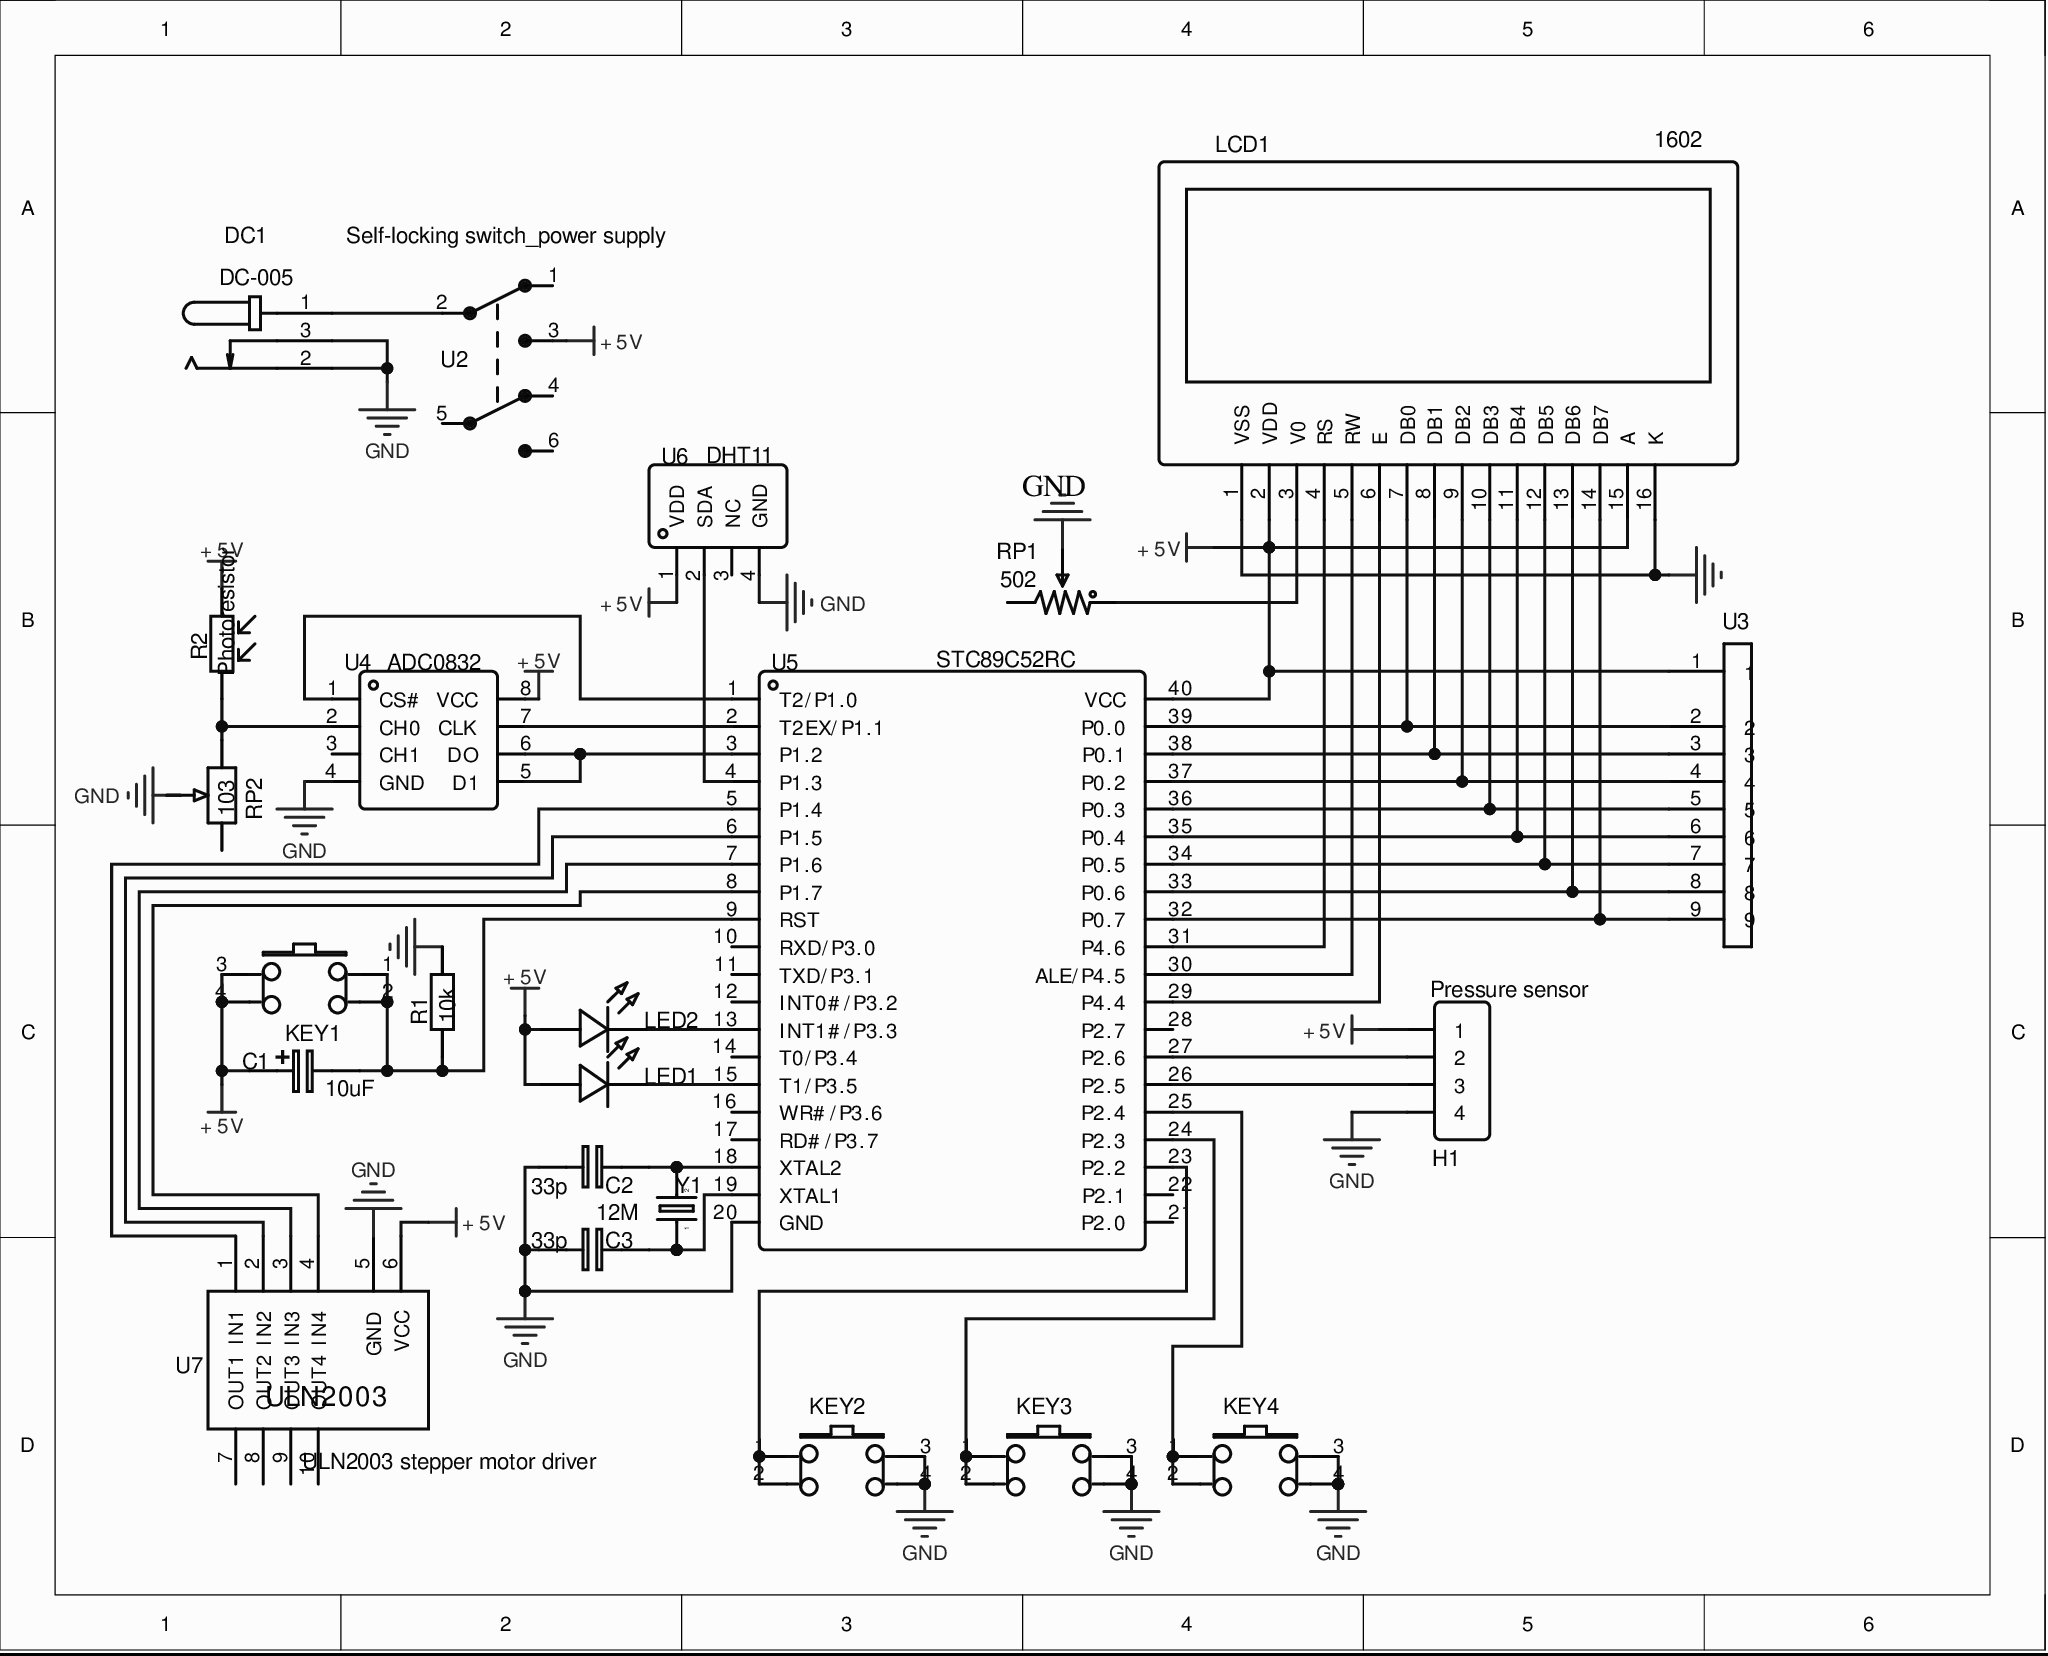
[diagram p0: MISC80828-9.schdoc]
# Altium project MISC80828-7.PrjPcb
1 sheet, 23 parts. Net scope: global (net labels, ports and power ports of the same name join across sheets).
Board file: MISC80828.PcbDoc

## Sheet MISC80828-9.schdoc
size 188 x 152 mm

### Parts
C1  10uF  [RB7.6-15]
C2  33p  [RAD-0.1]
C3  33p  [RAD-0.1]
DC1  DC-005  [DC-005]
H1  Pressure sensor  [HDR1X4]
KEY1  button6*6*8.5  [四脚轻触开关]  (value not drawn)
KEY2  button6*6*8.5  [四脚轻触开关]  (value not drawn)
KEY3  button6*6*8.5  [四脚轻触开关]  (value not drawn)
KEY4  button6*6*8.5  [四脚轻触开关]  (value not drawn)
LED1  LED-0603_R  [LED3MM]  (value not drawn)
LED2  LED-0603_R  [LED3MM]  (value not drawn)
R1  10k  [AXIAL-0.3]
R2  Photoresistor  [AXIAL-0.6]
RP1  502  [电位器]
RP2  103  [RM065]
U1  1602  [LCD1602]
U2  Self-locking switch_power supply  [自锁开关]
U3  respack-8  [HDR1X9]  (value not drawn)
U4  ADC0832  [DIP-8]
U5  STC89C52RC  [DIP40]
U6  DHT11  [HDR1X4]
U7  ULN2003 stepper motor driver  [ULN2003]
Y1  12M  [R38]

### Nets
+5V: C1.1 H1.1 KEY1.3 KEY1.4 LED1.1 LED2.1 R2.1 U1.2(VDD) U1.15(A) U2.3 U3.1 U4.8(VCC) U5.40(VCC) U6.1(VDD) U7.6(VCC)
GND: C2.1 C3.1 DC1.2 DC1.3 H1.4 KEY2.3 KEY2.4 KEY3.3 KEY3.4 KEY4.3 KEY4.4 R1.2 RP1.2 RP2.2 U1.1(VSS) U1.16(K) U4.4(GND) U5.20(GND) U6.4(GND) U7.5(GND)
NetC1_2: C1.2 KEY1.1 KEY1.2 R1.1 U5.9(RST)
NetC2_2: C2.2 U5.18(XTAL2) Y1.2
NetC3_2: C3.2 U5.19(XTAL1) Y1.1
NetDC1_1: DC1.1 U2.2
NetH1_2: H1.2 U5.27(P2.6)
NetH1_3: H1.3 U5.26(P2.5)
NetKEY2_1: KEY2.1 KEY2.2 U5.23(P2.2)
NetKEY3_1: KEY3.1 KEY3.2 U5.24(P2.3)
NetKEY4_1: KEY4.1 KEY4.2 U5.25(P2.4)
NetLED1_2: LED1.2 U5.13(INT1#/P3.3)
NetLED2_2: LED2.2 U5.15(T1/P3.5)
NetR2_2: R2.2 RP2.3 U4.2(CH0)
NetRP1_1: RP1.1 U1.3(V0)
NetU1_4: U1.4(RS) U5.31(P4.6)
NetU1_5: U1.5(RW) U5.30(ALE/P4.5)
NetU1_6: U1.6(E) U5.29(P4.4)
NetU1_7: U1.7(DB0) U3.2 U5.39(P0.0)
NetU1_8: U1.8(DB1) U3.3 U5.38(P0.1)
NetU1_9: U1.9(DB2) U3.4 U5.37(P0.2)
NetU1_10: U1.10(DB3) U3.5 U5.36(P0.3)
NetU1_11: U1.11(DB4) U3.6 U5.35(P0.4)
NetU1_12: U1.12(DB5) U3.7 U5.34(P0.5)
NetU1_13: U1.13(DB6) U3.8 U5.33(P0.6)
NetU1_14: U1.14(DB7) U3.9 U5.32(P0.7)
NetU4_1: U4.1(CS#) U5.1(T2/P1.0)
NetU4_5: U4.5(D1) U4.6(DO) U5.3(P1.2)
NetU4_7: U4.7(CLK) U5.2(T2EX/P1.1)
NetU5_4: U5.4(P1.3) U6.2(SDA)
NetU5_5: U5.5(P1.4) U7.1(IN1)
NetU5_6: U5.6(P1.5) U7.2(IN2)
NetU5_7: U5.7(P1.6) U7.3(IN3)
NetU5_8: U5.8(P1.7) U7.4(IN4)

Not connected (* = marked no-connect by the designer): RP1 3; RP2 1; U2 1 4 5 6; U4 3(CH1); U5 10(RXD/P3.0) 11(TXD/P3.1) 12(INT0#/P3.2) 14(T0/P3.4) 16(WR#/P3.6) 17(RD#/P3.7) 21(P2.0) 22(P2.1) 28(P2.7); U6 3(NC); U7 7(OUT1) 8(OUT2) 9(OUT3) 10(OUT4)

### Notes on the sheet
- (near RP1) GND

### Library data of the parts
C1 = 10uF: nameAlias: Value(F); Manufacturer Part: ?; spicePre: C; spiceSymbolName: Capacitor
C2 C3 = 33p: nameAlias: Value(F); spicePre: C; spiceSymbolName: Cap_RAD-0.1_EU
DC1 = DC-005: Manufacturer: XKB Enterprise; Manufacturer Part: DC-005-2.5A-2.0; Contributor: LCSC; Supplier: LCSC; Supplier Part: C319099; spicePre: D; spiceSymbolName: DC-005
H1 = 气压传感器: Contributor: LCEDA_Lib; Supplier Part: C225501; Supplier: LCSC; spicePre: H; spiceSymbolName: HDR-F-2.54_1x4
KEY1-KEY4 = button6*6*8.5: Manufacturer: ReliaPro; Supplier Part: C59980; Supplier: LCSC; Manufacturer Part: button6*6*8.5; spicePre: K; spiceSymbolName: button6*6*8.5
LED1 LED2 = LED-0603_R: Manufacturer: EVERLIGHT(台湾亿光); Manufacturer Part: 19-217/R6C-AL1M2VY/3T; Contributor: LCEDA_01; Supplier Part: C72044; Supplier: LCSC; spicePre: L; spiceSymbolName: LED-0603_R
R1 = 10k: nameAlias: Value(Ω); Manufacturer Part: ?; spicePre: R; spiceSymbolName: Resistor
R2 = 光敏: Manufacturer: Senba; Manufacturer Part: GL5516; nameAlias: Value; Contributor: lmytdxs; Supplier: LCSC; Supplier Part: C125626; spicePre: R; spiceSymbolName: GL5516
RP1 = 502: nameAlias: Value; Contributor: LCEDA_Lib; value(Ω): 10K; Supplier: LCSC; spicePre: R; spiceSymbolName: R_3386P_US
RP2 = 103: nameAlias: Resistance (Ohms); Contributor: LCEDA_Lib; Value(Ω): 10K; Supplier: LCSC; spicePre: R; spiceSymbolName: R_3386P_EU
U1 = 1602: Contributor: yybcc; spicePre: U; spiceSymbolName: 1602
U2 = 自锁开关_电源供电: Contributor: PERSON_A; Supplier Part: undefined; spicePre: U; spiceSymbolName: Self-locking switch_6 pin
U3 = respack-8: Contributor: dongguai; Manufacturer Part: respack-8; spicePre: U; spiceSymbolName: respack-8
U4 = ADC0832: Contributor: fghcd1; spicePre: U; spiceSymbolName: ADC0832
U5 = STC89C52RC: Manufacturer: STC; Manufacturer Part: STC89C52RC-40I; Supplier: LCSC; image: C14022.jpg; Supplier Part: C14022; spicePre: U; spiceSymbolName: STC89C52RC-40I
U6 = DHT11: Manufacturer: CYBERSEN(西博臣); Manufacturer Part: CHT11; Contributor: LCSC; Supplier: LCSC; Supplier Part: C476208; JLCPCB Part Class: Extended Part; spicePre: U; spiceSymbolName: CHT11
U7 = ULN2003步进电机驱动: Contributor: HBUTGYJ; spicePre: U; spiceSymbolName: ULN2003 motor driver
Y1 = 12M: Manufacturer Part: 49S8M; sourceId: ge82ICwN5; Supplier Part: 306010033; Supplier: SeeedStudio; timeStamp: 1476197612; spicePre: Y; spiceSymbolName: Crystal oscillator